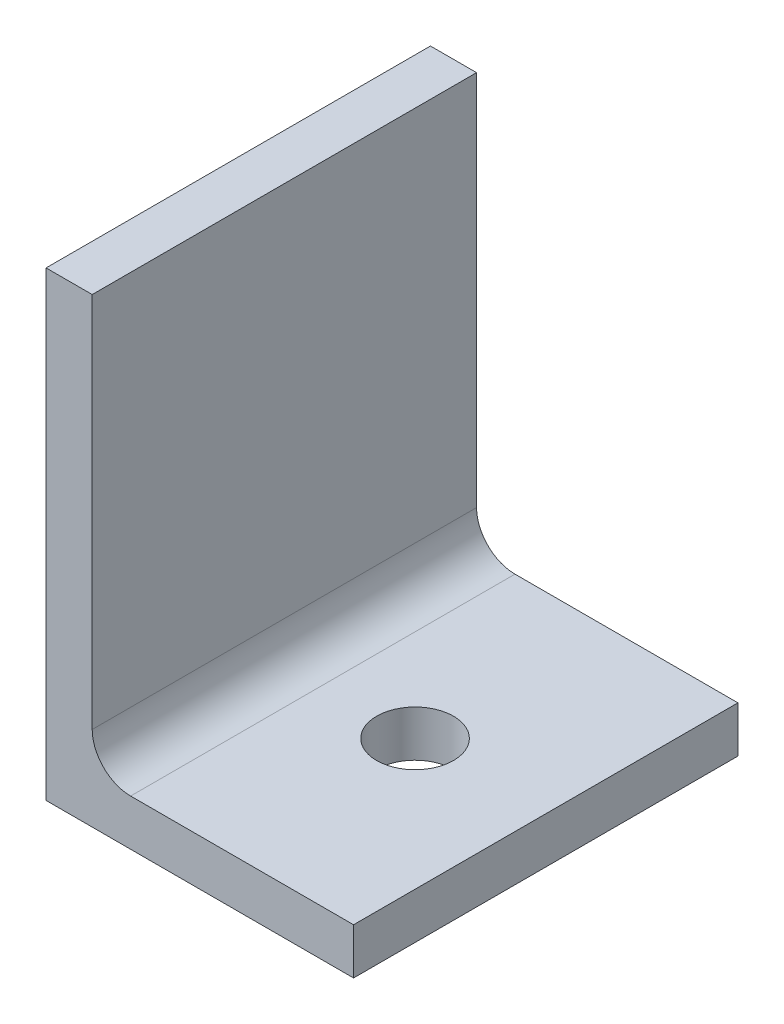
from build123d import *

# Parameters (mm, degrees)
BOSS_EXTRUDE1_DEPTH = 100
SKETCH2_R           = 10
CUT_EXTRUDE1_DEPTH  = 100


with BuildPart() as part:
    # Sketch1 → Boss-Extrude1 (new body)
    with BuildSketch(Plane.XY):
        with BuildLine():
            Line((0, 0), (0, -120))
            Line((0, -120), (80, -120))
            Line((80, -120), (80, -108))
            Line((80, -108), (22, -108))
            ThreePointArc((22, -108), (14.928932188, -105.071067812), (12, -98))
            Line((12, -98), (12, 0))
            Line((12, 0), (0, 0))
        make_face()
    extrude(amount=BOSS_EXTRUDE1_DEPTH)

    # Sketch2 → Cut-Extrude1 (cut)
    with BuildSketch(Plane(origin=(0, -108, 0), x_dir=(1, 0, 0), z_dir=(0, 1, 0))):
        with Locations(Location((46, -50, 0), (0, 0, 270))):
            Circle(SKETCH2_R)
    extrude(amount=-CUT_EXTRUDE1_DEPTH, mode=Mode.SUBTRACT)


solid = part.part
